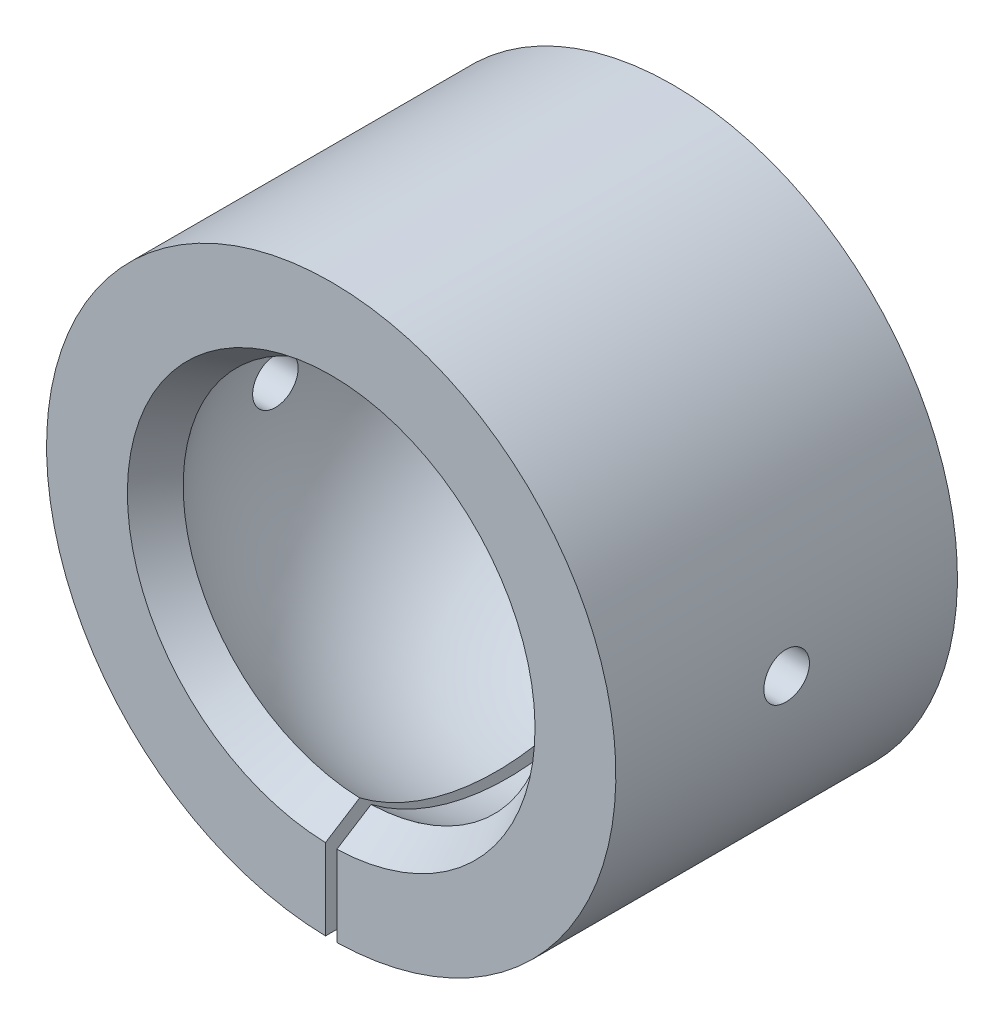
SolidWorks part; units mm, degrees
material "1.7035 (41Cr4)"
ref_plane "Front Plane" through (0, 0, 0) normal (0, 0, 1) x (1, 0, 0)
ref_plane "Top Plane" through (0, 0, 0) normal (0, 1, 0) x (1, 0, 0)
ref_plane "Right Plane" through (0, 0, 0) normal (1, 0, 0) x (0, 0, -1)
sketch "Sketch1" plane through (0, 0, 0) normal (0, 1, 0) x (1, 0, 0)
  line L0 (0, 23.6294) -> (0, -25.9558) construction
  line L1 (-25.3289, 0) -> (19.5175, 0) construction
  line L2 (17.9, -15) -> (16, -12)
  line L3 (13.2288, 15) -> (25, 15)
  line L5 (17.9, -15) -> (25, -15)
  line L6 (25, 15) -> (25, -15)
  arc A1 (16, -12) -> (13.2288, 15) centre (0, 0) ccw
  dimension "D3" = 20
  dimension "D1" = 50
  dimension "D2" = 30
  dimension "D4" = 32
  dimension "D5" = 35.8
revolve "Revolve1" add sketch "Sketch1" angle 360 about L0
sketch "Sketch2" plane through (0, 0, 0) normal (0, 1, 0) x (1, 0, 0)
  line L0 (-42.0549, 0) -> (39.4178, 0) construction
  line L1 (0, 42.9571) -> (0, -41.708) construction
  line L5 (-0.5, 17.5) -> (0.5, 17.5)
  line L6 (-0.5, 17.5) -> (-0.5, -17.5)
  line L7 (-0.5, -17.5) -> (0.5, -17.5)
  line L8 (0.5, 17.5) -> (0.5, -17.5)
  dimension "D1" = 35
  dimension "D2" = 1
extrude "Cut-Extrude1" cut sketch "Sketch2" against normal through all
sketch "Sketch3" plane through (0, 0, 0) normal (1, 0, 0) x (0, 0, -1)
  circle A0 centre (0, 0) radius 2
  dimension "D1" = 4
extrude "Cut-Extrude2" cut sketch "Sketch3" against normal through all both and the other way through all
